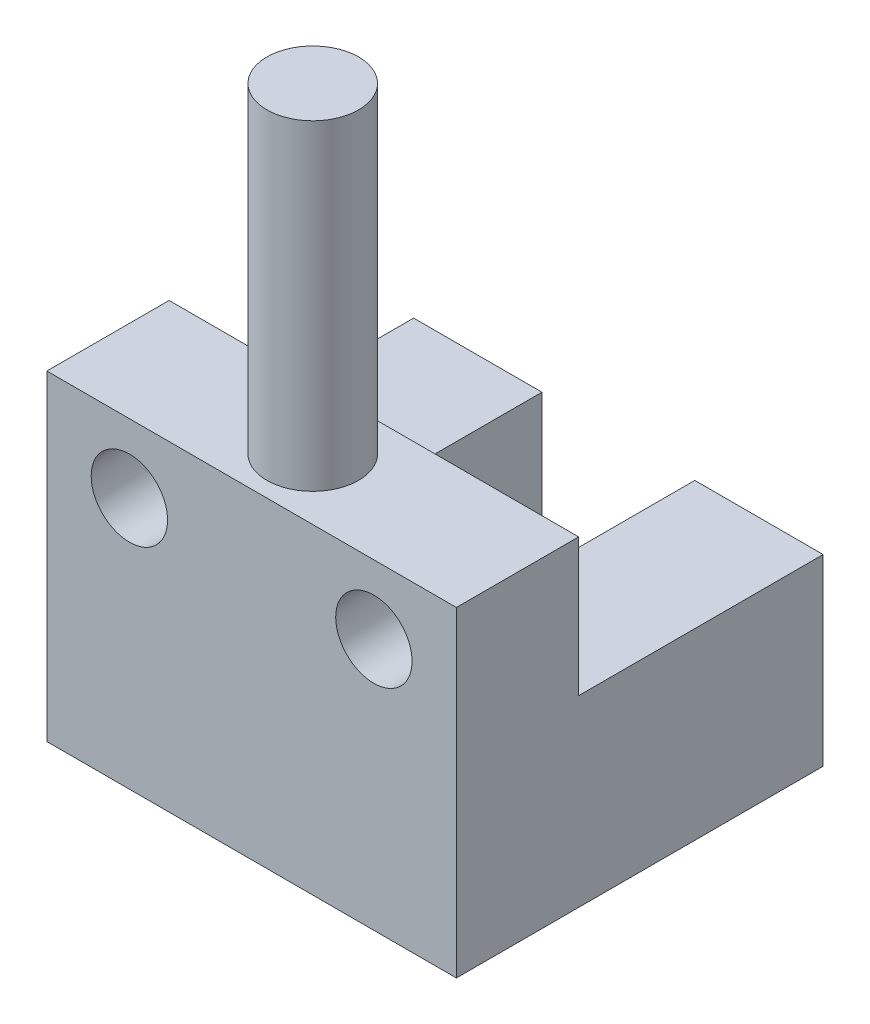
SolidWorks part; units mm, degrees
ref_plane "Front Plane" through (0, 0, 0) normal (0, 0, 1) x (1, 0, 0)
ref_plane "Top Plane" through (0, 0, 0) normal (0, 1, 0) x (1, 0, 0)
ref_plane "Right Plane" through (0, 0, 0) normal (1, 0, 0) x (0, 0, -1)
sketch "Sketch1" plane through (0, 0, 0) normal (0, 1, 0) x (1, 0, 0)
  line L0 (2.5, 6) -> (6.7, 6)
  line L1 (-6.7, 6) -> (-2.5, 6)
  line L2 (-6.7, 6) -> (-6.7, -6)
  line L3 (-6.7, -6) -> (6.7, -6)
  line L4 (6.7, 6) -> (6.7, -6)
  line L5 (-6.7, 6) -> (6.7, -6) construction
  line L6 (-6.7, -6) -> (6.7, 6) construction
  line L7 (0, 6) -> (0, 50006) construction
  line L8 (-2.5, 6) -> (-2.5, 0.5)
  line L9 (-2.5, 0.5) -> (2.5, 0.5)
  line L10 (2.5, 6) -> (2.5, 0.5)
  line L11 (-2.5, 11.5) -> (2.5, 0.5) construction
  line L12 (-2.5, 0.5) -> (2.5, 11.5) construction
  point P0 (0, 0)
  point P6 (0, 6)
  dimension "D1" = 13.4
  dimension "D2" = 12
  dimension "D3" = 5.5
  dimension "D4" = 5
extrude "Boss-Extrude1" add sketch "Sketch1" along normal blind 6
sketch "Sketch2" plane through (0, 6, 0) normal (0, 1, 0) x (1, 0, 0)
  line L0 (-6.7, 6) -> (-6.7, -6) construction
  line L1 (-6.7, -6) -> (6.7, -6)
  line L2 (-6.7, -6) -> (-6.7, -2)
  line L3 (-6.7, -2) -> (6.7, -2)
  line L4 (6.7, -6) -> (6.7, -2)
  line L5 (6.7, -6) -> (6.7, 6) construction
  line L6 (-6.7, -6) -> (6.7, -6) construction
  dimension "D1" = 4
extrude "Boss-Extrude2" add sketch "Sketch2" along normal blind 4.5
sketch "Sketch3" plane through (0, 10.5, 0) normal (0, 1, 0) x (1, 0, 0)
  line L0 (0, 0) -> (0, 50000) construction
  line L1 (-6.7, -4) -> (49993.3, -4) construction
  line L2 (-6.7, -2) -> (-6.7, -6) construction
  circle A0 centre (0, -4) radius 1.5
  point P7 (-6.7, -4)
  dimension "D1" = 3
extrude "Boss-Extrude3" add sketch "Sketch3" along normal blind 10.5
sketch "Sketch4" plane through (0, 0, 2) normal (0, 0, -1) x (-1, 0, 0)
  line L0 (0, 0) -> (0, 50000) construction
  line L1 (6.7, 8.25) -> (-49993.3, 8.25) construction
  line L2 (6.7, 10.5) -> (6.7, 6) construction
  circle A0 centre (-4, 8.25) radius 1.25
  circle A1 centre (4, 8.25) radius 1.25
  point P7 (6.7, 8.25)
  dimension "D1" = 8
  dimension "D2" = 2.5
extrude "Cut-Extrude1" cut sketch "Sketch4" against normal blind 10.5
sketch "Sketch5" plane through (2.5, 0, 0) normal (-1, 0, 0) x (0, 0, 1)
  line L0 (-6, 3) -> (49994, 3) construction
  line L1 (-6, 6) -> (-6, 0) construction
  line L2 (6, 10.5) -> (6, 0) construction
  circle A0 centre (-4, 3) radius 0.5
  point P4 (-6, 3)
  dimension "D1" = 1
  dimension "D2" = 10
extrude "Boss-Extrude4" add sketch "Sketch5" along normal up to surface (5 mm away) up to face at (-2.5, 3, -3.25)
